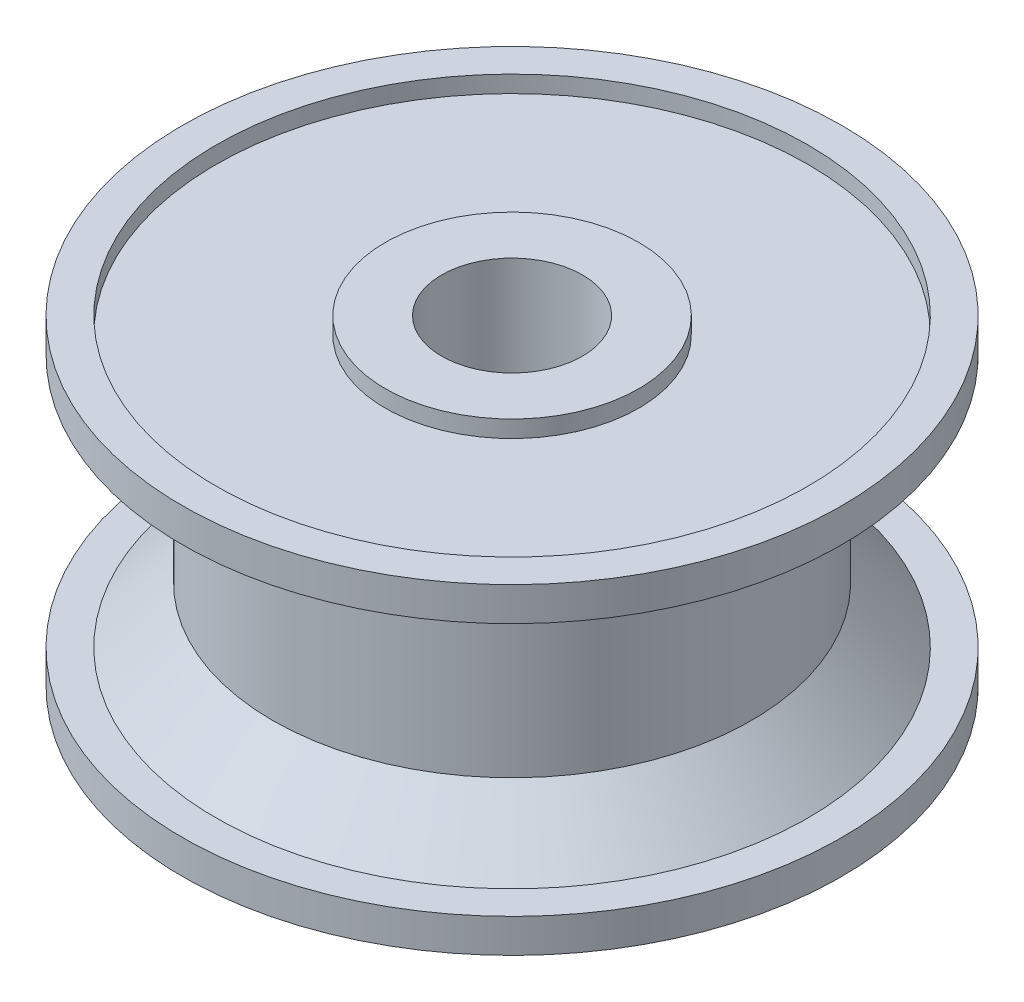
from build123d import *

# Parameters (mm, degrees)
SKETCH_2_R          = 12.5
CUT_EXTRUDE_1_DEPTH = 101.466412298
SKETCH_3_R          = 52.5
SKETCH_3_R_2        = 22.5
CUT_EXTRUDE_2_DEPTH = 3


with BuildPart() as part:
    # 草图1 → 旋转1 (revolve)
    with BuildSketch(Plane.XY, mode=Mode.PRIVATE) as revolve_1_sk:
        Polygon((52.5, 22.5), (58.5, 22.5), (58.5, 28.5), (0, 28.5), (0, -28.5), (58.5, -28.5), (58.5, -22.5), (52.5, -22.5), (42.5, -12.5), (42.5, 12.5), align=None)
    revolve(revolve_1_sk.sketch.rotate(Axis((0, -28.5, 0), (0, 1, 0)), 90), axis=Axis((0, -28.5, 0), (0, 1, 0)))

    # 草图2 → 切除-拉伸1 (cut, through all)
    with BuildSketch(Plane.XZ.offset(28.5)):
        with Locations(Location((0, 0, 0), (0, 0, 270))):
            Circle(SKETCH_2_R)
    extrude(amount=-CUT_EXTRUDE_1_DEPTH, mode=Mode.SUBTRACT)

    # 草图3 → 切除-拉伸2 (cut)
    with BuildSketch(Plane.XZ.offset(28.5)):
        with Locations(Location((0, 0, 0), (0, 0, 270))):
            Circle(SKETCH_3_R)
        with Locations(Location((0, 0, 0), (0, 0, 270))):
            Circle(SKETCH_3_R_2, mode=Mode.SUBTRACT)
    cut_extrude_2 = extrude(amount=-CUT_EXTRUDE_2_DEPTH, mode=Mode.SUBTRACT)

    # 镜向1: 切除-拉伸2 across plane
    add(cut_extrude_2.mirror(Plane.ZX), mode=Mode.SUBTRACT)


solid = part.part
